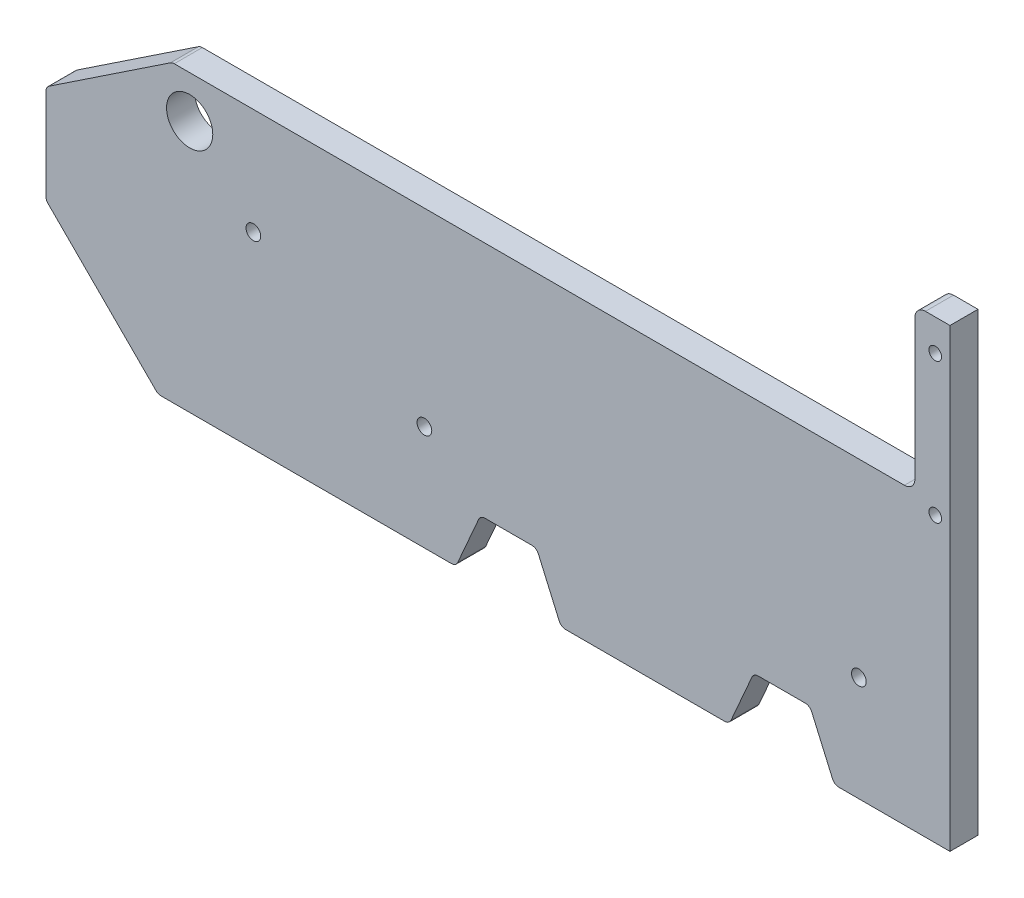
SolidWorks part; units mm, degrees
material "Q235B"
ref_plane "Front Plane" through (0, 0, 0) normal (0, 0, 1) x (1, 0, 0)
ref_plane "Top Plane" through (0, 0, 0) normal (0, 1, 0) x (1, 0, 0)
ref_plane "Right Plane" through (0, 0, 0) normal (1, 0, 0) x (0, 0, -1)
sketch "Sketch1" plane through (0, 0, 0) normal (0, 0, 1) x (1, 0, 0)
  line L0 (1240, 420) -> (1240, 650)
  line L1 (0, 0) -> (1290, 0)
  line L2 (0, 0) -> (0, 420)
  line L3 (0, 420) -> (1240, 420)
  line L4 (1290, 0) -> (1290, 650)
  line L5 (1240, 650) -> (1290, 650)
  circle A0 centre (205, 360) radius 33
  circle A1 centre (1269, 405) radius 9
  circle A2 centre (1269, 605) radius 9
  dimension "D3" = 360
  dimension "D5" = 66
  dimension "D4" = 1085
  dimension "D13" = 18
  dimension "D14" = 21
  dimension "D8" = 18
  dimension "D9" = 200
  dimension "D10" = 21
  dimension "D11" = 405
  dimension "D1" = 1290
  dimension "D2" = 50
  dimension "D6" = 420
  dimension "D7" = 230
extrude "Boss-Extrude1" add sketch "Sketch1" along normal blind 40
chamfer "Chamfer2" distance 180 distance2 120 1 edges at (0, 420, 20)
chamfer "Chamfer3" distance 160 angle 45 1 edges at (0, 0, 20)
sketch "Sketch2" plane through (0, 0, 40) normal (0, 0, 1) x (1, 0, 0)
  line L0 (585, 0) -> (735, 0)
  line L1 (160, 0) -> (1290, 0) construction
  line L3 (620, 80) -> (700, 80)
  line L5 (975, 0) -> (1125, 0)
  line L6 (1090, 80) -> (1125, 0)
  line L7 (1010, 80) -> (1090, 80)
  line L8 (1010, 80) -> (975, 0)
  line L9 (1240, 420) -> (180, 420) construction
  line L10 (1290, 0) -> (1290, 650) construction
  line L12 (700, 80) -> (735, 0)
  line L13 (620, 80) -> (585, 0)
  dimension "D1" = 340
  dimension "D2" = 200
  dimension "D3" = 590
  dimension "D4" = 80
  dimension "D5" = 80
  dimension "D6" = 150
  dimension "D7" = 35
  dimension "D8" = 150
  dimension "D9" = 35
hole_wizard "M24 Tapped Hole1" positions "3DSketch1" profile "Sketch3" tap size "M24" standard "GB" end condition up to next
sketch3d "3DSketch1"
  line L6 (160, 0, 40) -> (1290, 0, 40) construction
  point P13 (540, 150, 40)
  point P15 (1160, 150, 40)
  point P27 (295.9354, 268.3163, 40)
  dimension "D4" = 150
  dimension "D7" = 150
sketch "Sketch3" plane through (540, 150, 40) normal (1, 0, 0) x (0, -1, 0)
  line L0 (0, 0) -> (0, 40)
  line L1 (0, 40) -> (10.5, 40)
  line L2 (10.5, 40) -> (10.5, 0)
  line L5 (10.5, 0) -> (0, 0)
  line L11 (0, -6.35) -> (0, 107.95) construction
  dimension "通孔螺纹孔钻头直径" = 21
  dimension "通孔螺纹孔钻头深度" = 40
cosmetic thread "Hole thread 3" parameters "D2"=24
cosmetic thread "Hole thread 4" parameters "D2"=24
cosmetic thread "Hole thread 5" parameters "D2"=24
fillet "Fillet1" radius 15 2 edges at (1240, 420, 20) (1240, 650, 20)
extrude "Cut-Extrude1" cut sketch "Sketch2" against normal through all
fillet "Fillet2" radius 10 8 edges at (1010, 80, 20) (1090, 80, 20) (1125, 0, 20) (975, 0, 20) (700, 80, 20) (620, 80, 20) (735, 0, 20) (585, 0, 20)
fillet "Fillet3" radius 10 4 edges at (160, 0, 20) (0, 160, 20) (0, 300, 20) (180, 420, 20)
